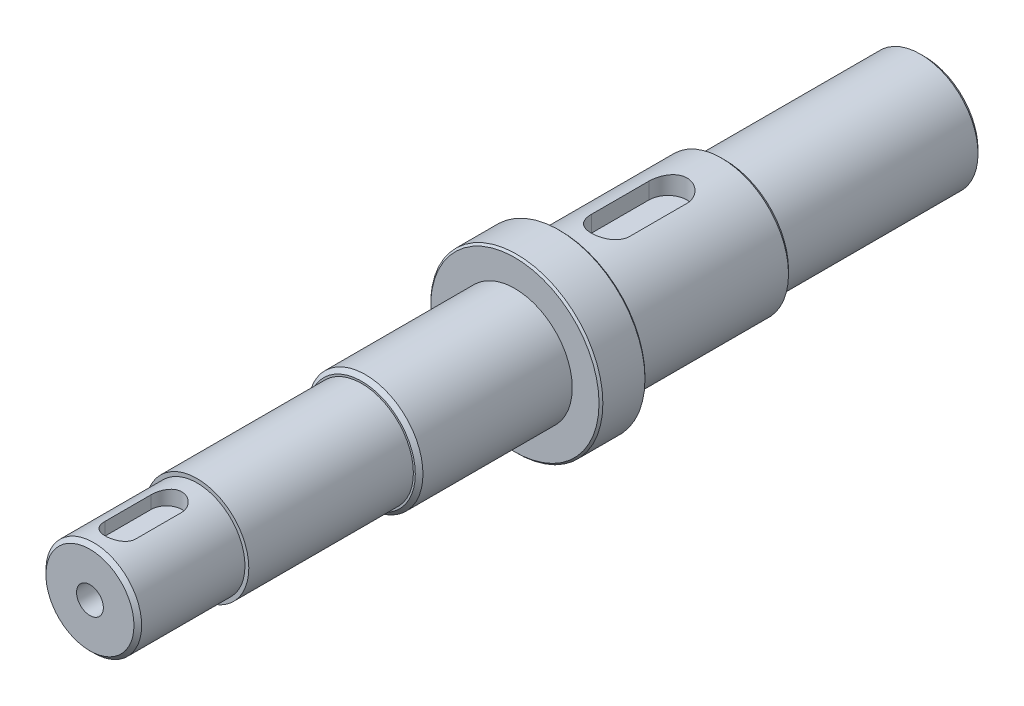
from build123d import *

# Parameters (mm, degrees)
SKETCH1_R                 = 15
BOSS_EXTRUDE1_DEPTH       = 52
SKETCH2_R                 = 17.5
BOSS_EXTRUDE2_DEPTH       = 43
SKETCH3_R                 = 22.5
BOSS_EXTRUDE3_DEPTH       = 12
SKETCH4_R                 = 15
BOSS_EXTRUDE4_DEPTH       = 40
SKETCH5_R                 = 13.5
BOSS_EXTRUDE5_DEPTH       = 43
SKETCH6_R                 = 12.5
BOSS_EXTRUDE6_DEPTH       = 28
CHAMFER1_SIZE             = 1
CHAMFER2_SIZE             = 1
CHAMFER3_SIZE             = 0.5
CUT_EXTRUDE1_START        = 12.5
CUT_EXTRUDE1_DEPTH        = 20
CUT_EXTRUDE2_START        = 8.5
CUT_EXTRUDE2_DEPTH        = 10
M8X1_0_TAPPED_HOLE1_D     = 7
M8X1_0_TAPPED_HOLE1_DEPTH = 19
M8X1_0_TAPPED_HOLE1_TIP   = 2.103012167


with BuildPart() as part:
    # Sketch1 → Boss-Extrude1 (new body)
    with BuildSketch(Plane.XY):
        with Locations(Location((0, 0, 0), (0, 0, 180))):
            Circle(SKETCH1_R)
    extrude(amount=BOSS_EXTRUDE1_DEPTH)

    # Sketch2 → Boss-Extrude2 (add)
    with BuildSketch(Plane.XY.offset(52)):
        Circle(SKETCH2_R)
    extrude(amount=BOSS_EXTRUDE2_DEPTH)

    # Sketch3 → Boss-Extrude3 (add)
    with BuildSketch(Plane.XY.offset(95)):
        Circle(SKETCH3_R)
    extrude(amount=BOSS_EXTRUDE3_DEPTH)

    # Sketch4 → Boss-Extrude4 (add)
    with BuildSketch(Plane.XY.offset(107)):
        with Locations(Location((0, 0, 0), (0, 0, 180))):
            Circle(SKETCH4_R)
    extrude(amount=BOSS_EXTRUDE4_DEPTH)

    # Sketch5 → Boss-Extrude5 (add)
    with BuildSketch(Plane.XY.offset(147)):
        Circle(SKETCH5_R)
    extrude(amount=BOSS_EXTRUDE5_DEPTH)

    # Sketch6 → Boss-Extrude6 (add)
    with BuildSketch(Plane.XY.offset(190)):
        Circle(SKETCH6_R)
    extrude(amount=BOSS_EXTRUDE6_DEPTH)

    # Chamfer1
    chamfer1_edges = [part.edges().sort_by_distance(p)[0] for p in [
        (15, 0, 0),
    ]]
    chamfer(chamfer1_edges, length=CHAMFER1_SIZE)

    # Chamfer2
    chamfer2_edges = [part.edges().sort_by_distance(p)[0] for p in [
        (15, 0, 147),
        (-12.5, 0, 218),
        (-17.5, 0, 52),
    ]]
    chamfer(chamfer2_edges, length=CHAMFER2_SIZE)

    # Chamfer3
    chamfer3_edges = [part.edges().sort_by_distance(p)[0] for p in [
        (-22.5, 0, 95),
        (-22.5, 0, 107),
    ]]
    chamfer(chamfer3_edges, length=CHAMFER3_SIZE)

    # Sketch7 → Cut-Extrude1 (cut)
    with BuildSketch(Plane(origin=(0, 0, 0), x_dir=(1, 0, 0), z_dir=(0, 1, 0)).offset(CUT_EXTRUDE1_START)):
        with BuildLine():
            Line((5, -67), (5, -82))
            ThreePointArc((5, -82), (0, -87), (-5, -82))
            Line((-5, -82), (-5, -67))
            ThreePointArc((-5, -67), (0, -62), (5, -67))
        make_face()
    extrude(amount=CUT_EXTRUDE1_DEPTH, mode=Mode.SUBTRACT)

    # Sketch8 → Cut-Extrude2 (cut)
    with BuildSketch(Plane(origin=(0, 0, 0), x_dir=(1, 0, 0), z_dir=(0, 1, 0)).offset(CUT_EXTRUDE2_START)):
        with BuildLine():
            Line((4, -198), (4, -210))
            ThreePointArc((4, -210), (0, -214), (-4, -210))
            Line((-4, -210), (-4, -198))
            ThreePointArc((-4, -198), (0, -194), (4, -198))
        make_face()
    extrude(amount=CUT_EXTRUDE2_DEPTH, mode=Mode.SUBTRACT)

    # M8x1.0 Tapped Hole1
    with Locations(Plane.XY.offset(218)):
        with Locations((0, 0)):
            Hole(M8X1_0_TAPPED_HOLE1_D / 2, depth=M8X1_0_TAPPED_HOLE1_DEPTH)
            with Locations((0, 0, -(M8X1_0_TAPPED_HOLE1_DEPTH + M8X1_0_TAPPED_HOLE1_TIP / 2))):  # 118° drill point
                Cone(0, M8X1_0_TAPPED_HOLE1_D / 2, M8X1_0_TAPPED_HOLE1_TIP, mode=Mode.SUBTRACT)


solid = part.part
